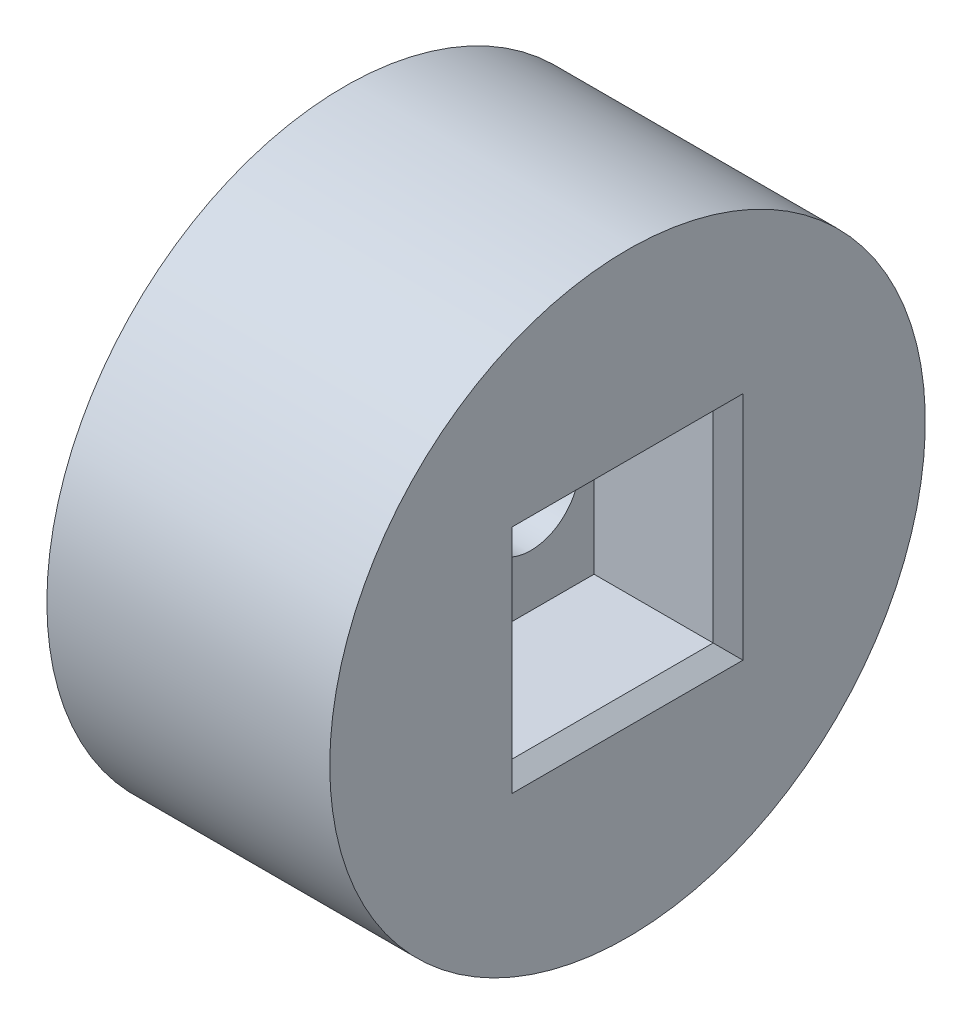
SolidWorks part; units mm, degrees
ref_plane "Front" through (0, 0, 0) normal (0, 0, 1) x (1, 0, 0)
ref_plane "Top" through (0, 0, 0) normal (0, 1, 0) x (1, 0, 0)
ref_plane "Right" through (0, 0, 0) normal (1, 0, 0) x (0, 0, -1)
sketch "Sketch1" plane through (0, 0, 0) normal (0, 1, 0) x (1, 0, 0)
  line L0 (0, 0) -> (22.8061, 0) construction
  line L2 (0, 0) -> (19, 0)
  line L3 (0, 0) -> (0, -20)
  line L4 (0, -20) -> (19, -20)
  line L5 (19, 0) -> (19, -20)
  dimension "D1" = 40
  dimension "D2" = 19
revolve "Revolve1" add sketch "Sketch1" angle 360 about L0
sketch "Sketch2" plane through (19, 0, 0) normal (1, 0, 0) x (0, 0, -1)
  line L1 (6.75, -6.75) -> (-6.75, -6.75)
  line L2 (6.75, -6.75) -> (6.75, 6.75)
  line L3 (6.75, 6.75) -> (-6.75, 6.75)
  line L4 (-6.75, -6.75) -> (-6.75, 6.75)
  line L5 (6.75, -6.75) -> (-6.75, 6.75) construction
  line L6 (6.75, 6.75) -> (-6.75, -6.75) construction
  point P0 (0, 0)
  dimension "D1" = 13.5
extrude "Cut-Extrude1" cut sketch "Sketch2" against normal blind 9
hole_wizard "CBORE for M3 Hex Socket Head Cap Screw1" positions "Sketch4" profile "Sketch3" counterbore size "M3" standard "ISO" end condition through all
sketch "Sketch4" plane through (10, 0, 0) normal (1, 0, 0) x (0, 0, -1)
  point P0 (2.5, 0)
  dimension "D1" = 2.5
sketch "Sketch3" plane through (10, 0, -2.5) normal (0, 1, 0) x (0, 0, -1)
  line L0 (0, 0) -> (0, 10)
  line L1 (0, 10) -> (1.7, 10)
  line L3 (1.7, 10) -> (1.7, 3.5)
  line L4 (1.7, 3.5) -> (3.25, 3.5)
  line L5 (3.25, 3.5) -> (3.25, 0)
  line L7 (3.25, 0) -> (0, 0)
  line L11 (0, -6.35) -> (0, 107.95) construction
  dimension "Thru Hole Dia." = 3.4
  dimension "Thru Hole Depth" = 10
  dimension "C'Bore Dia." = 6.5
  dimension "C'Bore Depth" = 3.5
sketch "Sketch5" plane through (10, 0, 0) normal (1, 0, 0) x (0, 0, -1)
  line L0 (-2, 0) -> (-4, 0) construction
  line L1 (-2, -1) -> (-4, -1)
  line L2 (-2, 1) -> (-4, 1)
  arc A0 (-2, -1) -> (-2, 1) centre (-2, 0) ccw
  arc A1 (-4, 1) -> (-4, -1) centre (-4, 0) ccw
  point P3 (-3, 0)
  dimension "D3" = 1
  dimension "D1" = 2
  dimension "D2" = 2
extrude "Cut-Extrude2" cut sketch "Sketch5" against normal through all
sketch "Sketch6" plane through (0, 0, 0) normal (-1, 0, 0) x (0, 0, 1)
  circle A0 centre (0, 0) radius 5.2
  dimension "D1" = 10.4
extrude "Cut-Extrude3" cut sketch "Sketch6" against normal blind 3
chamfer "Chamfer1" distance 0.5 angle 45 1 edges at (0, 0, 5.2)
chamfer "Chamfer2" distance 1 angle 45 4 edges at (19, 0, -6.75) (19, -6.75, 0) (19, 0, 6.75) (19, 6.75, 0)
